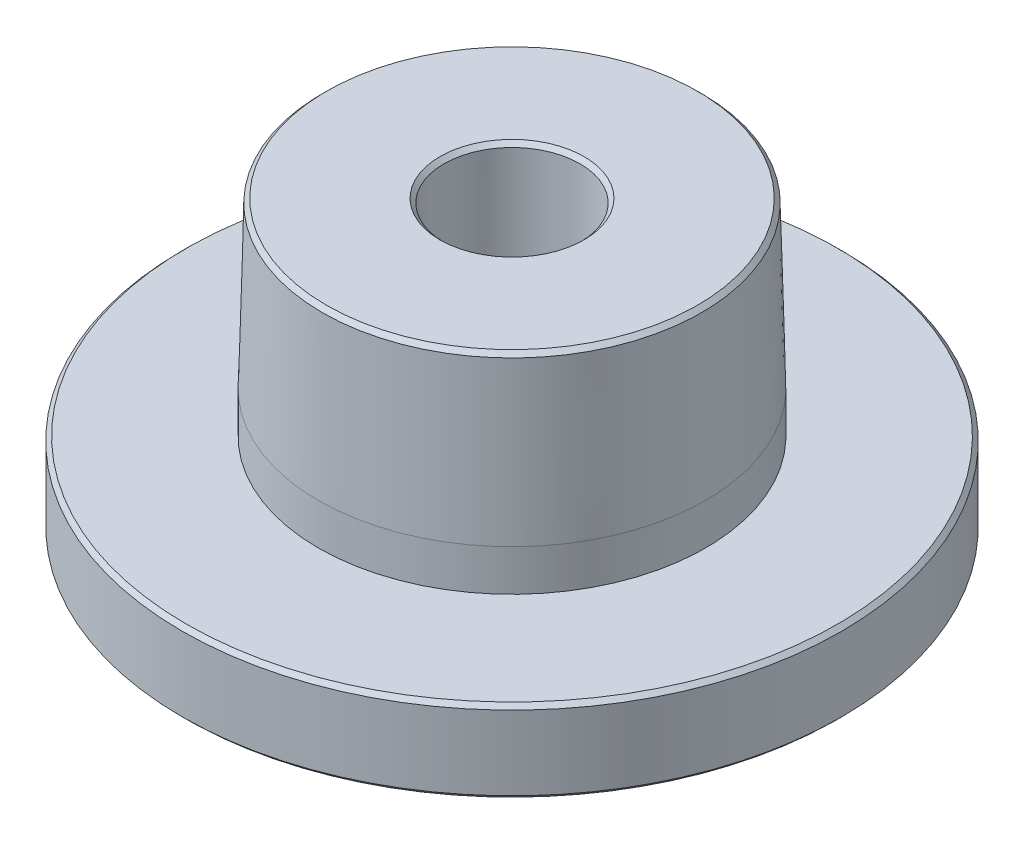
from build123d import *
from OCP.BRepFilletAPI import BRepFilletAPI_MakeChamfer

# Parameters (mm, degrees)
CHAMFER1_SIZE  = 0.5
CHAMFER1_SIZE2 = 0.512980744


with BuildPart() as part:
    # Sketch1 → Revolve1 (revolve)
    with BuildSketch(Plane.XY, mode=Mode.PRIVATE) as revolve1_sk:
        Polygon((8.25, 35), (23, 35), (23.5, 15), (23.5, 10), (40, 10), (40, 0), (8.25, 0), align=None)
    revolve(revolve1_sk.sketch.rotate(Axis((0, 0, 0), (0, 1, 0)), 90), axis=Axis((0, 0, 0), (0, 1, 0)))

    # Chamfer1: one chamfer whose edges measure the first distance from different faces: ONE call of the kernel's chamfer builder (chamfer() names one face for all edges)
    chamfer1_edges_1 = [part.edges().sort_by_distance(p)[0] for p in [
        (0, 10, 40),
        (0, 0, 40),
        (0, 0, 8.25),
        (0, 35, 8.25),
    ]]
    chamfer1_edges_2 = [part.edges().sort_by_distance(p)[0] for p in [
        (0, 35, 23),
    ]]
    chamfer1_side_2 = [part.faces().sort_by_distance(p)[0] for p in [
        (0, 35, 8.900538239),
    ]]
    chamfer1 = BRepFilletAPI_MakeChamfer(part.part.solid().wrapped)
    for e in chamfer1_edges_1:
        chamfer1.Add(CHAMFER1_SIZE, e.wrapped)
    for e in chamfer1_edges_2:
        chamfer1.Add(CHAMFER1_SIZE, CHAMFER1_SIZE2, e.wrapped, chamfer1_side_2[0].wrapped)  # the first distance lies on this face
    add(Compound.cast(chamfer1.Shape()), mode=Mode.REPLACE)


solid = part.part
